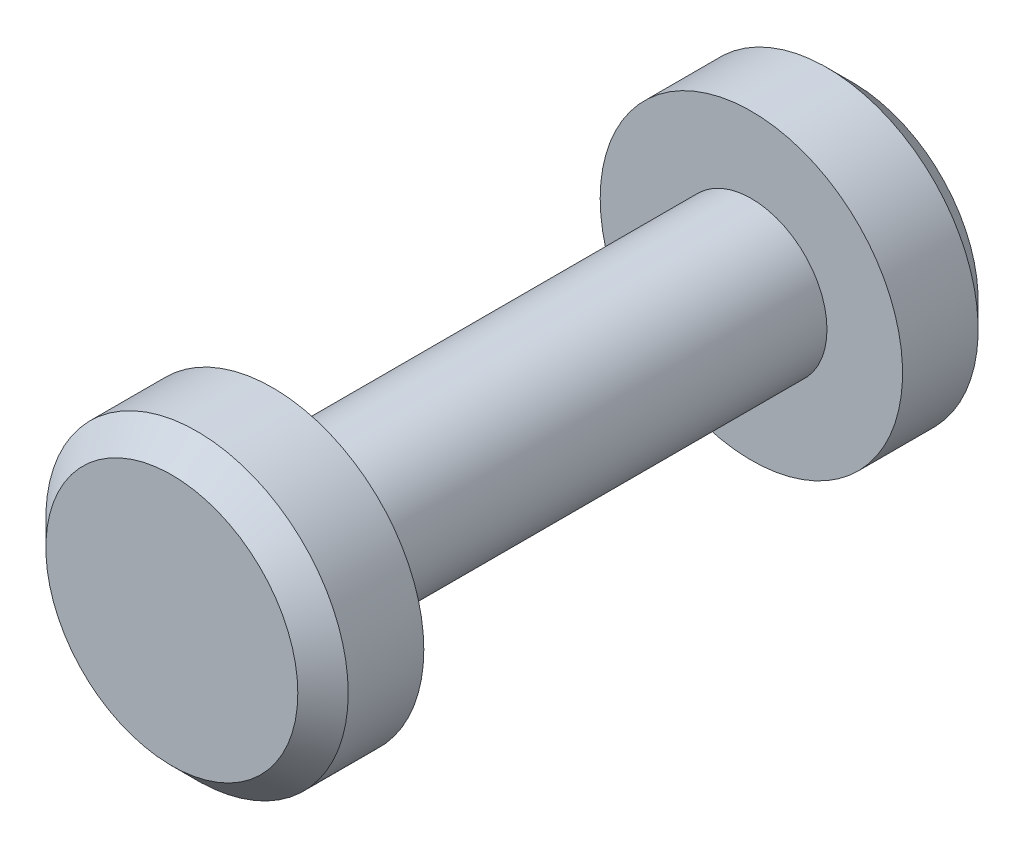
from build123d import *

# Parameters (mm, degrees)
SKETCH_1_R      = 3
EXTRUDE_1_DEPTH = 19
SKETCH_2_R      = 6
EXTRUDE_2_DEPTH = 4
CHAMFER_1_SIZE  = 1
EXTRUDE_START   = 4
SKETCH_3_R      = 6
EXTRUDE_3_DEPTH = 4
CHAMFER_2_SIZE  = 1


with BuildPart() as part:
    # 草图1 → 凸台-拉伸1 (new body)
    with BuildSketch(Plane.XY):
        Circle(SKETCH_1_R)
    extrude(amount=EXTRUDE_1_DEPTH)

    # 草图2 → 凸台-拉伸2 (add)
    with BuildSketch(Plane.XY.offset(19)):
        Circle(SKETCH_2_R)
    extrude(amount=EXTRUDE_2_DEPTH)

    # 倒角1
    chamfer_1_edges = [part.edges().sort_by_distance(p)[0] for p in [
        (-6, 0, 23),
    ]]
    chamfer(chamfer_1_edges, length=CHAMFER_1_SIZE)

    # 草图3 → 凸台-拉伸3 (add)
    with BuildSketch(Plane(origin=(0, 0, 0), x_dir=(-1, 0, 0), z_dir=(0, 0, -1)).offset(EXTRUDE_START)):
        with Locations(Location((0, 0, 0), (0, 0, 180))):
            Circle(SKETCH_3_R)
    extrude(amount=-EXTRUDE_3_DEPTH)

    # 倒角2
    chamfer_2_edges = [part.edges().sort_by_distance(p)[0] for p in [
        (-6, 0, -4),
    ]]
    chamfer(chamfer_2_edges, length=CHAMFER_2_SIZE)


solid = part.part
